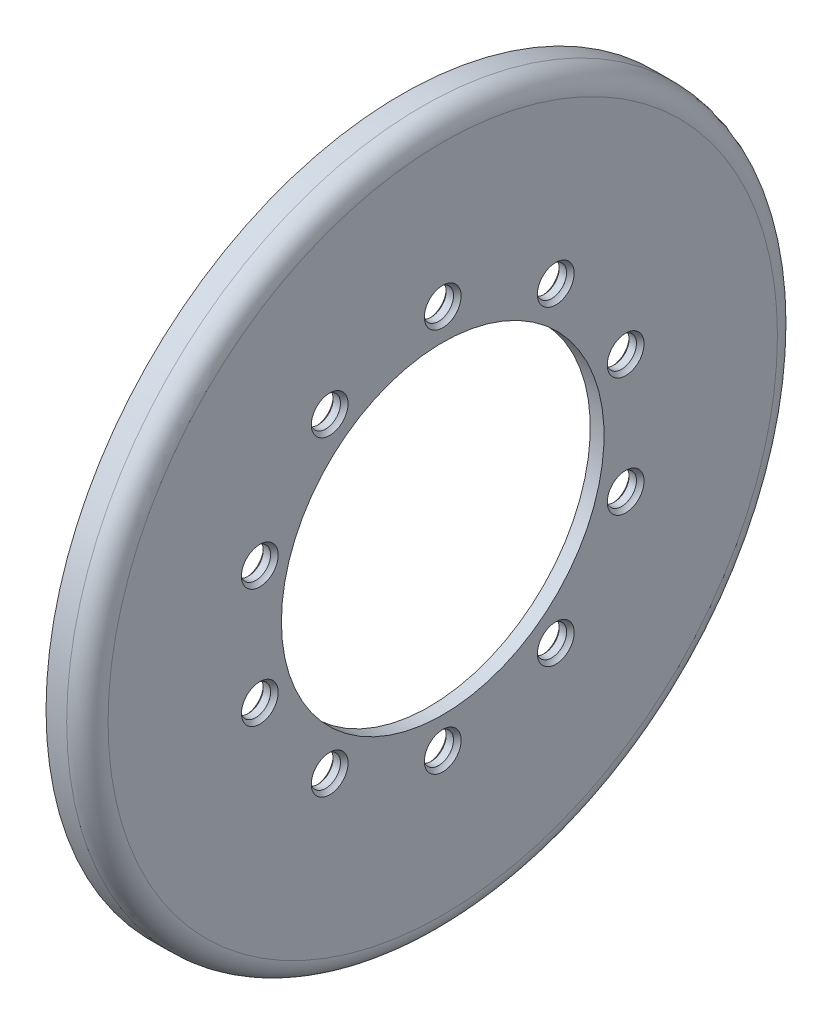
from build123d import *

# Parameters (mm, degrees)
FILLET_1_R                           = 18
FILLET_2_R                           = 4
SKETCH_2_R                           = 13
CUT_EXTRUDE_1_DEPTH                  = 440.177071421
CHAMFER_1_SIZE                       = 2
PATTERN_CIRCULAR_1_COUNT             = 10
CHAMFER_1_OF_PATTERN_CIRCULAR_1_SIZE = 2


with BuildPart() as part:
    # 草图1 → 旋转1 (revolve)
    with BuildSketch(Plane.XY, mode=Mode.PRIVATE) as revolve_1_sk:
        Polygon((0, 309.5), (36, 309.5), (36, 140.5), (24, 140.5), (24, 217.5), (22, 217.5), (22, 295.5), (0, 295.5), align=None)
    revolve(revolve_1_sk.sketch.rotate(Axis((-295.4, 0, 0), (1, 0, 0)), 90), axis=Axis((-295.4, 0, 0), (1, 0, 0)))

    # 圆角1
    fillet_1_edges = [part.edges().sort_by_distance(p)[0] for p in [
        (36, 0, -309.5),
    ]]
    fillet(fillet_1_edges, radius=FILLET_1_R)

    # 圆角2
    fillet_2_edges = [part.edges().sort_by_distance(p)[0] for p in [
        (22, 0, -295.5),
    ]]
    fillet(fillet_2_edges, radius=FILLET_2_R)

    # 草图2 → 切除-拉伸1 (cut, through all)
    with BuildSketch(Plane(origin=(36, 0, 0), x_dir=(0, 0, -1), z_dir=(1, 0, 0))):
        with Locations((0, 167.5)):
            Circle(SKETCH_2_R)
    cut_extrude_1 = extrude(amount=-CUT_EXTRUDE_1_DEPTH, mode=Mode.SUBTRACT)

    # 倒角1
    chamfer_1_edges = [part.edges().sort_by_distance(p)[0] for p in [
        (24, 167.5, 13),
    ]]
    chamfer(chamfer_1_edges, length=CHAMFER_1_SIZE)

    # 草图3 → 切除-旋转1 (revolve, cut)
    with BuildSketch(Plane.XY, mode=Mode.PRIVATE) as cut_revolve_1_sk:
        with BuildLine():
            Line((32.398120874, 180.50807098), (32.398120874, 167.5))
            Line((32.398120874, 167.5), (65.246950766, 167.5))
            ThreePointArc((65.246950766, 167.5), (53.242386137, 185.165329999), (32.398120874, 180.50807098))
        make_face()
    cut_revolve_1 = revolve(cut_revolve_1_sk.sketch.rotate(Axis((0, 167.5, 0), (1, 0, 0)), 270), axis=Axis((0, 167.5, 0), (1, 0, 0)), mode=Mode.SUBTRACT)

    # 阵列(圆周)1: 切除-拉伸1, 切除-旋转1 ×10 about axis
    pattern_circular_1_axis = Axis((0, 0, 0), (1, 0, 0))
    add([cut_extrude_1.rotate(pattern_circular_1_axis, i * 360 / PATTERN_CIRCULAR_1_COUNT) for i in range(1, PATTERN_CIRCULAR_1_COUNT)], mode=Mode.SUBTRACT)
    add([cut_revolve_1.rotate(pattern_circular_1_axis, i * 360 / PATTERN_CIRCULAR_1_COUNT) for i in range(1, PATTERN_CIRCULAR_1_COUNT)], mode=Mode.SUBTRACT)

    # 倒角1 of 阵列(圆周)1
    chamfer_1_of_pattern_circular_1_edges = [part.edges().sort_by_distance(p)[0] for p in [
        (24, 127.869138278, 108.971250686),
        (24, 39.396611846, 163.319187406),
        (24, -64.12408127, 155.284745553),
        (24, -143.151554838, 87.936808832),
        (24, -167.5, -13),
        (24, -127.869138278, -108.971250686),
        (24, -39.396611846, -163.319187406),
        (24, 64.12408127, -155.284745553),
        (24, 143.151554838, -87.936808832),
    ]]
    chamfer(chamfer_1_of_pattern_circular_1_edges, length=CHAMFER_1_OF_PATTERN_CIRCULAR_1_SIZE)


solid = part.part
